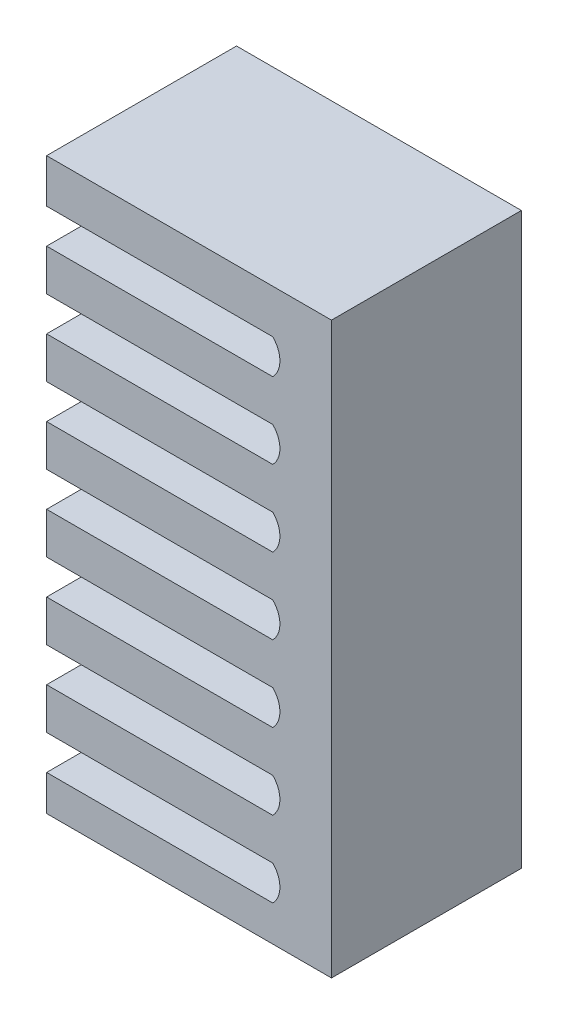
SolidWorks part; units mm, degrees
ref_plane "前视基准面" through (0, 0, 0) normal (0, 0, 1) x (1, 0, 0)
ref_plane "上视基准面" through (0, 0, 0) normal (0, 1, 0) x (1, 0, 0)
ref_plane "右视基准面" through (0, 0, 0) normal (1, 0, 0) x (0, 0, -1)
other "Configuration Table"
sketch "草图1" plane through (0, 0, 0) normal (0, 0, 1) x (1, 0, 0)
  line L0 (7.5, -15) -> (-7.5, -15)
  line L1 (7.5, -15) -> (7.5, 15)
  line L2 (7.5, 15) -> (-7.5, 15)
  line L3 (-7.5, -15) -> (-7.5, -13.1259)
  line L4 (-7.5, -13.1259) -> (4.4073, -13.1259)
  line L5 (4.4073, -7.3044) -> (-7.5, -7.3044)
  line L6 (4.4073, -11.3044) -> (-7.5, -11.3044)
  line L7 (-7.5, -9.1259) -> (4.4073, -9.1259)
  line L8 (4.4073, -3.3044) -> (-7.5, -3.3044)
  line L9 (-7.5, -5.1259) -> (4.4073, -5.1259)
  line L10 (4.4073, 0.6956) -> (-7.5, 0.6956)
  line L11 (-7.5, -1.1259) -> (4.4073, -1.1259)
  line L12 (4.4073, 4.6956) -> (-7.5, 4.6956)
  line L13 (-7.5, 2.8741) -> (4.4073, 2.8741)
  line L14 (4.4073, 8.6956) -> (-7.5, 8.6956)
  line L15 (-7.5, 6.8741) -> (4.4073, 6.8741)
  line L16 (4.4073, 12.6956) -> (-7.5, 12.6956)
  line L17 (-7.5, 10.8741) -> (4.4073, 10.8741)
  line L18 (-7.5, 12.6956) -> (-7.5, 15)
  line L19 (-7.5, -11.3044) -> (-7.5, -9.1259)
  line L20 (-7.5, -7.3044) -> (-7.5, -5.1259)
  line L21 (-7.5, -3.3044) -> (-7.5, -1.1259)
  line L22 (-7.5, 0.6956) -> (-7.5, 2.8741)
  line L23 (-7.5, 6.8741) -> (-7.5, 4.6956)
  line L24 (-7.5, 8.6956) -> (-7.5, 10.8741)
  arc A0 (4.4073, -13.1259) -> (4.4073, -11.3044) centre (3.4966, -12.2151) ccw
  arc A1 (4.4073, -9.1259) -> (4.4073, -7.3044) centre (3.4966, -8.2151) ccw
  arc A2 (4.4073, -5.1259) -> (4.4073, -3.3044) centre (3.4966, -4.2151) ccw
  arc A3 (4.4073, -1.1259) -> (4.4073, 0.6956) centre (3.4966, -0.2151) ccw
  arc A4 (4.4073, 2.8741) -> (4.4073, 4.6956) centre (3.4966, 3.7849) ccw
  arc A5 (4.4073, 6.8741) -> (4.4073, 8.6956) centre (3.4966, 7.7849) ccw
  arc A6 (4.4073, 10.8741) -> (4.4073, 12.6956) centre (3.4966, 11.7849) ccw
  dimension "D1" = 30
extrude "凸台-拉伸1" add sketch "草图1" along normal mid plane 10
